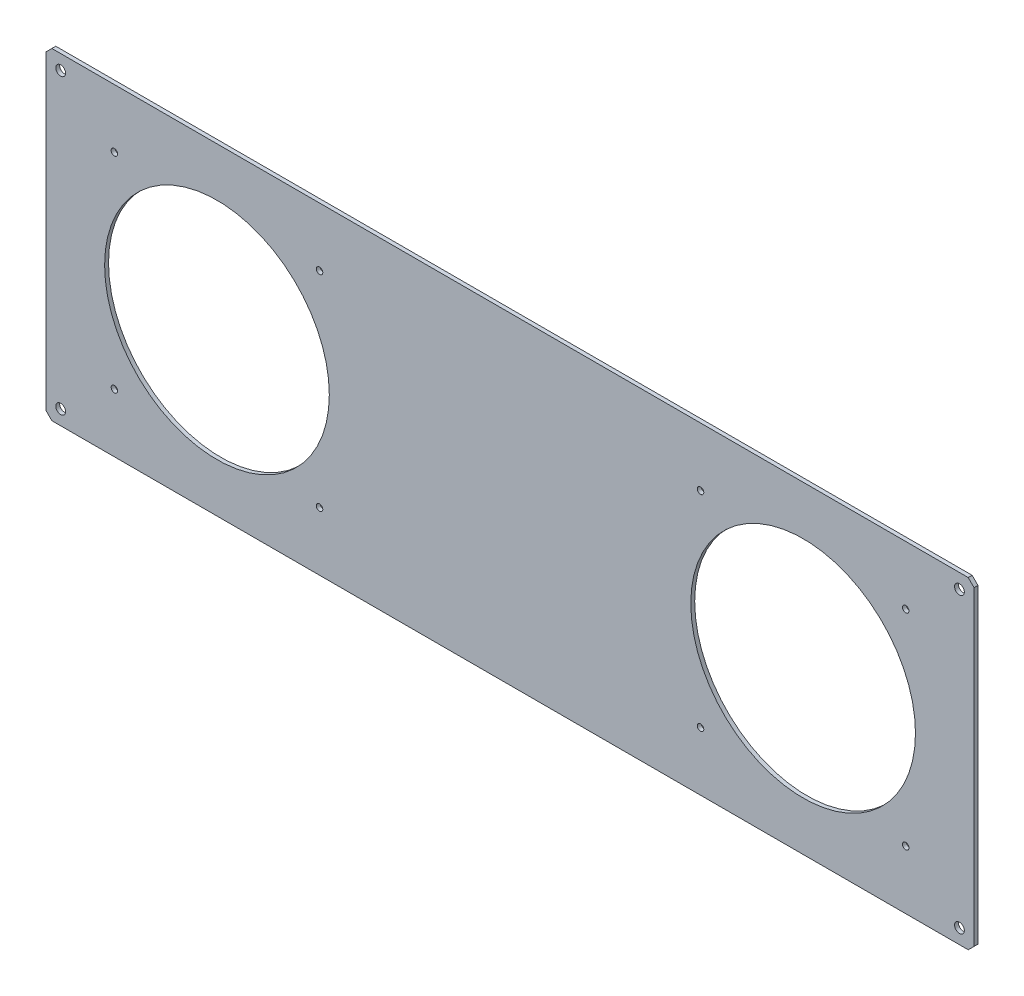
from build123d import *

# Parameters (mm, degrees)
SKETCH_1_W             = 475
SKETCH_1_H             = 165
EXTRUDE_1_DEPTH        = 2
HOLE_WIZARD_5_0_5_1_D  = 5
CHAMFER_1_SIZE         = 3
SKETCH_4_R             = 57.5
CUT_EXTRUDE_1_DEPTH    = 2
HOLE_WIZARD_M4_1_D     = 3.3
HOLE_WIZARD_M4_1_DEPTH = 10.1
HOLE_WIZARD_M4_1_TIP   = 0.991420021


with BuildPart() as part:
    # 草图1 → 凸台-拉伸1 (new body)
    with BuildSketch(Plane.XY):
        Rectangle(SKETCH_1_W, SKETCH_1_H)
    extrude(amount=EXTRUDE_1_DEPTH)

    # Ø5.0 (5) 直径孔1 (through all)
    with Locations(Plane.XY.offset(2)):
        with Locations((-230, 75), (-230, -75), (230, 75), (230, -75)):
            Hole(HOLE_WIZARD_5_0_5_1_D / 2)

    # 倒角1
    chamfer_1_edges = [part.edges().sort_by_distance(p)[0] for p in [
        (237.5, -82.5, 1),
        (-237.5, -82.5, 1),
        (-237.5, 82.5, 1),
        (237.5, 82.5, 1),
    ]]
    chamfer(chamfer_1_edges, length=CHAMFER_1_SIZE)

    # 草图4 → 切除-拉伸1 (cut)
    with BuildSketch(Plane.XY.offset(2)):
        with Locations((-150, 0)):
            Circle(SKETCH_4_R)
        with Locations((150, 0)):
            Circle(SKETCH_4_R)
    extrude(amount=-CUT_EXTRUDE_1_DEPTH, mode=Mode.SUBTRACT)

    # M4 螺纹孔1
    with Locations(Plane.XY.offset(2)):
        with Locations((-202.5, 52.5), (-97.5, 52.5), (-97.5, -52.5), (-202.5, -52.5), (97.5, -52.5), (202.5, -52.5), (202.5, 52.5), (97.5, 52.5)):
            Hole(HOLE_WIZARD_M4_1_D / 2, depth=HOLE_WIZARD_M4_1_DEPTH)
            with Locations((0, 0, -(HOLE_WIZARD_M4_1_DEPTH + HOLE_WIZARD_M4_1_TIP / 2))):  # 118° drill point
                Cone(0, HOLE_WIZARD_M4_1_D / 2, HOLE_WIZARD_M4_1_TIP, mode=Mode.SUBTRACT)


solid = part.part
